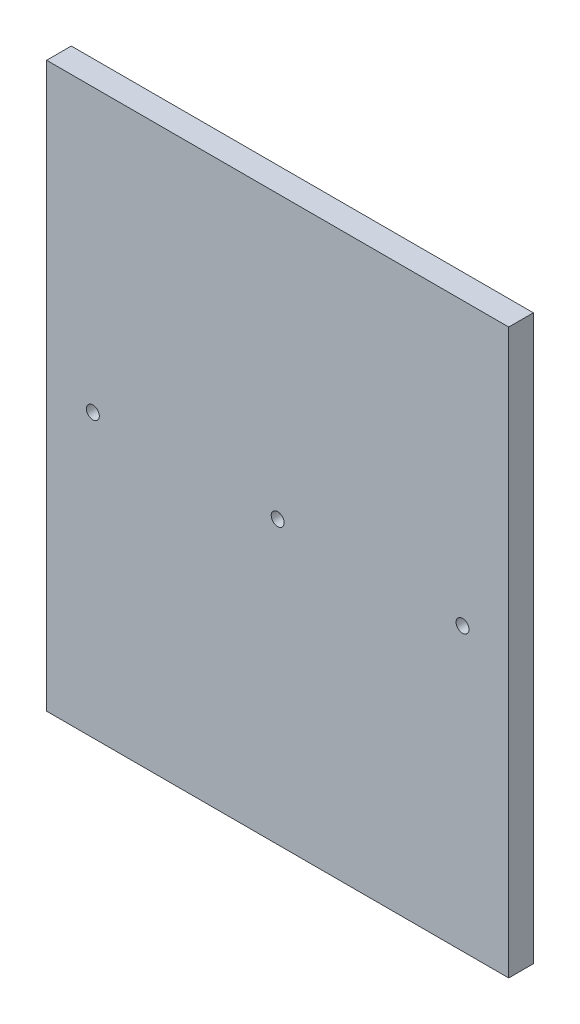
from build123d import *

# Parameters (mm, degrees)
SKETCH1_W           = 150
SKETCH1_H           = 183
BOSS_EXTRUDE1_DEPTH = 4
M5_TAPPED_HOLE1_D   = 4.2


with BuildPart() as part:
    # Sketch1 → Boss-Extrude1 (new, symmetric)
    with BuildSketch(Plane.XY):
        Rectangle(SKETCH1_W, SKETCH1_H)
    extrude(amount=BOSS_EXTRUDE1_DEPTH, both=True)

    # M5 Tapped Hole1 (through all)
    with Locations(Plane.XY.offset(4)):
        with Locations((-60, 0), (0, 0), (60, 0)):
            Hole(M5_TAPPED_HOLE1_D / 2)


solid = part.part
